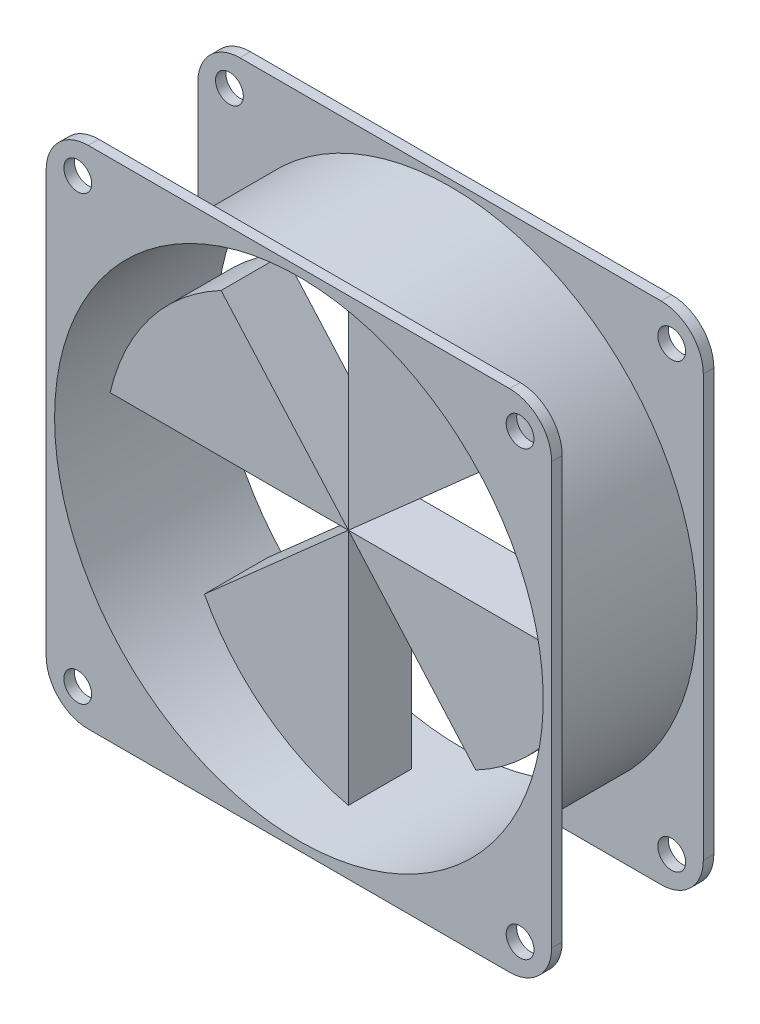
SolidWorks part; units mm, degrees
material "普通碳钢"
ref_plane "Front" through (0, 0, 0) normal (0, 0, 1) x (1, 0, 0)
ref_plane "Top" through (0, 0, 0) normal (0, 1, 0) x (1, 0, 0)
ref_plane "Right" through (0, 0, 0) normal (1, 0, 0) x (0, 0, -1)
sketch "草图1" plane through (0, 0, 0) normal (0, 0, 1) x (1, 0, 0)
  line L1 (-60, -60) -> (60, -60)
  line L2 (-60, -60) -> (-60, 60)
  line L3 (-60, 60) -> (60, 60)
  line L4 (60, -60) -> (60, 60)
  line L5 (-60, -60) -> (60, 60) construction
  line L6 (-60, 60) -> (60, -60) construction
  point P0 (0, 0)
  dimension "D1" = 120
  dimension "D2" = 120
extrude "凸台-拉伸1" add sketch "草图1" along normal blind 2.5
sketch "草图2" plane through (0, 0, 2.5) normal (0, 0, 1) x (1, 0, 0)
  circle A0 centre (0, 0) radius 58.5
  circle A1 centre (0, 0) radius 56.5
  dimension "D1" = 2
  dimension "D2" = 113
extrude "凸台-拉伸2" add sketch "草图2" along normal blind 33.5
sketch "草图4" plane through (0, 0, 0) normal (0, 0, -1) x (-1, 0, 0)
  circle A0 centre (0, 0) radius 58
extrude "切除-拉伸1" cut sketch "草图4" against normal through all
fillet "圆角1" radius 10 4 edges at (60, 60, 1.25) (60, -60, 1.25) (-60, -60, 1.25) (-60, 60, 1.25)
ref_plane "基准面1" through (0, 0, 19.25) normal (0, 0, 1) x (1, 0, 0)
mirror "镜向1" about plane through (0, 0, 19.25) normal (0, 0, 1) of "切除-拉伸1", "凸台-拉伸1", "圆角1"
sketch "草图6" plane through (0, 0, 19.25) normal (0, 0, 1) x (1, 0, 0)
  line L0 (0, 0) -> (0, 56.5676)
  line L1 (34.183, 30.2233) -> (0, 0)
  arc A0 (0, 56.5676) -> (34.183, 30.2233) centre (-11.6714, 6.0743) cw
extrude "凸台-拉伸3" add sketch "草图6" along normal mid plane 15 separate body
pattern_circular "阵列(圆周)2" count 4 every 90 about axis through (0, 0, 0) along (0, 0, 1) of bodies 105
hole_wizard "M6 间隙孔1" positions "草图8" profile "草图9" hole size "M6" standard "Gb" end condition through all
sketch "草图8" plane through (0, 0, 38.5) normal (0, 0, 1) x (1, 0, 0)
  line L0 (0, 0) -> (94.6543, 0) construction
  line L2 (0, 0) -> (0, 89.4263) construction
  point P0 (-52.5, 52.5)
  point P3 (52.5, 52.5)
  point P6 (52.5, -52.5)
  point P9 (-52.5, -52.5)
  dimension "D1" = 105
  dimension "D2" = 105
sketch "草图9" plane through (-52.5, 52.5, 38.5) normal (1, 0, 0) x (0, -1, 0)
  line L0 (0, 0) -> (0, 38.5)
  line L1 (0, 38.5) -> (3.3, 38.5)
  line L2 (3.3, 38.5) -> (3.3, 0)
  line L5 (3.3, 0) -> (0, 0)
  line L11 (0, -6.35) -> (0, 107.95) construction
  dimension "通孔孔直径" = 6.6
  dimension "通孔孔深度" = 38.5
